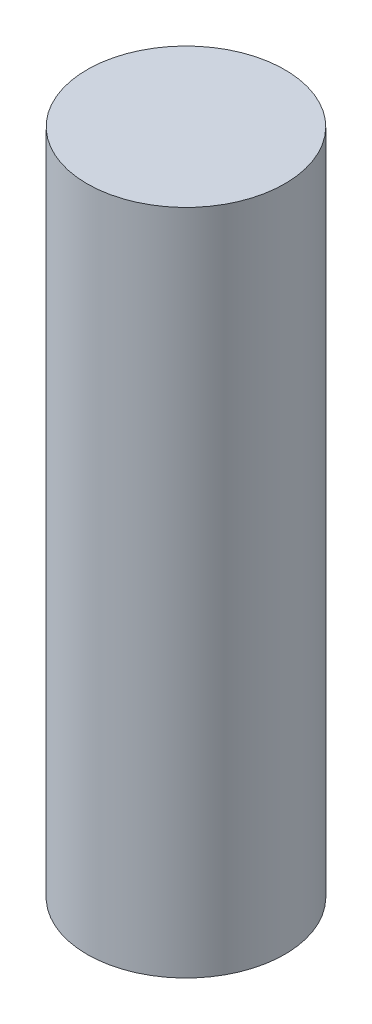
from build123d import *

# Parameters (mm, degrees)
SKETCH1_R           = 8
BOSS_EXTRUDE1_DEPTH = 54


with BuildPart() as part:
    # Sketch1 → Boss-Extrude1 (new body)
    with BuildSketch(Plane(origin=(0, 0, 0), x_dir=(1, 0, 0), z_dir=(0, 1, 0))):
        with Locations(Location((0, 0, 0), (0, 0, 270))):
            Circle(SKETCH1_R)
    extrude(amount=BOSS_EXTRUDE1_DEPTH)


solid = part.part
